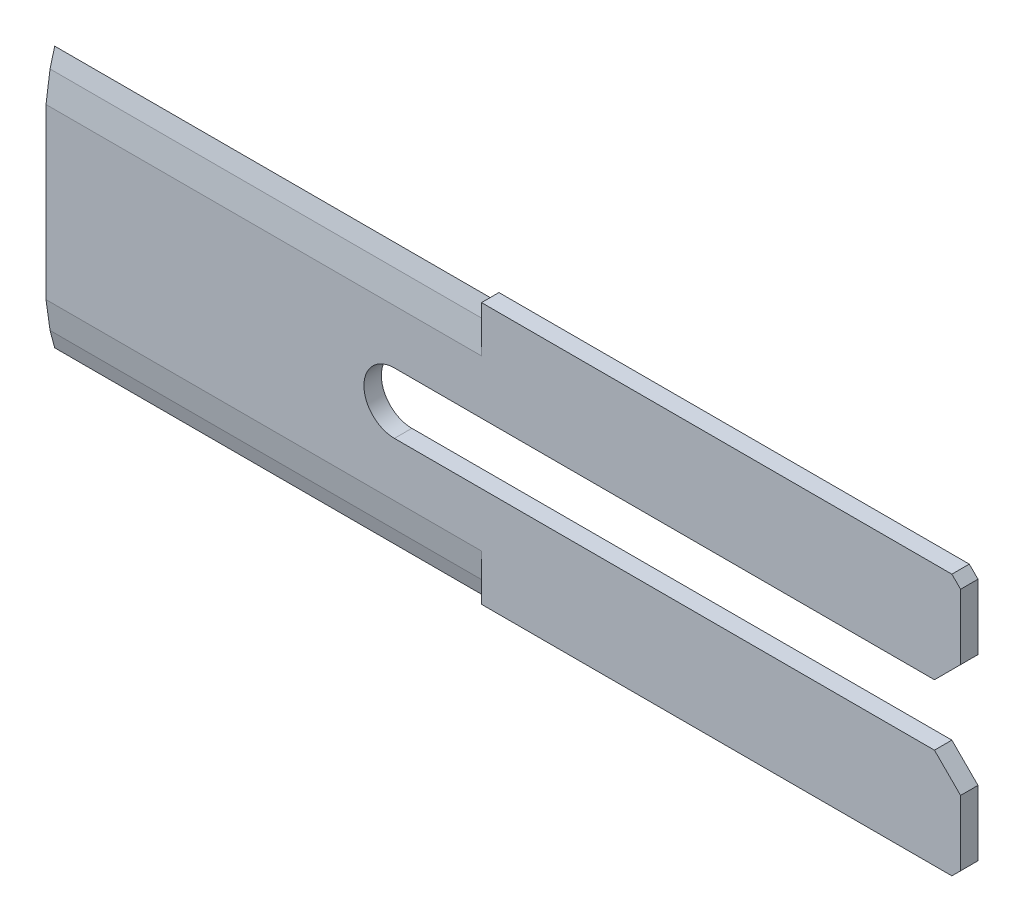
SolidWorks part; units mm, degrees
ref_plane "前视基准面" through (0, 0, 0) normal (0, 0, 1) x (1, 0, 0)
ref_plane "上视基准面" through (0, 0, 0) normal (0, 1, 0) x (1, 0, 0)
ref_plane "右视基准面" through (0, 0, 0) normal (1, 0, 0) x (0, 0, -1)
sketch "草图2" plane through (0, 0, 0) normal (0, 0, 1) x (1, 0, 0)
  line L1 (-52.5, 15) -> (52.5, 15)
  line L2 (-52.5, 15) -> (-52.5, -15)
  line L3 (-52.5, -15) -> (52.5, -15)
  line L4 (52.5, 15) -> (52.5, -15)
  line L5 (-52.5, 15) -> (52.5, -15) construction
  line L6 (-52.5, -15) -> (52.5, 15) construction
  point P0 (0, 0)
  dimension "D1" = 105
  dimension "D2" = 30
extrude "凸台-拉伸1" add sketch "草图2" along normal blind 2
sketch "草图3" plane through (0, 0, 2) normal (0, 0, 1) x (1, 0, 0)
  line L0 (-12.5, 3.5) -> (52.5, 3.5)
  line L1 (52.5, -15) -> (52.5, 15) construction
  line L2 (-12.5, -3.5) -> (52.5, -3.5)
  line L3 (52.5, 15) -> (-52.5, 15) construction
  arc A0 (-12.5, 3.5) -> (-12.5, -3.5) centre (-12.5, 0) ccw
  dimension "D1" = 7
  dimension "D2" = 65
  dimension "D3" = 15
extrude "切除-拉伸1" cut sketch "草图3" against normal through all and the other way through all
sketch "草图5" plane through (-52.5, 0, 0) normal (-1, 0, 0) x (0, 0, 1)
  line L0 (1, 16.6149) -> (1, -17.4095) construction
  line L1 (1, 15) -> (0.4641, 13)
  line L2 (2, 15) -> (0, 15) construction
  line L3 (1, 15) -> (1.5359, 13)
  line L4 (0, 9.6977) -> (0, -9.6977)
  line L5 (0.4641, 13) -> (0, 9.6977)
  line L6 (0, 15) -> (0, -15) construction
  line L7 (1.5359, 13) -> (2, 9.6977)
  line L8 (2, 15) -> (2, -15) construction
  line L9 (-0.6309, 0) -> (2.7776, 0) construction
  line L10 (1.5359, -13) -> (2, -9.6977)
  line L11 (0.4641, -13) -> (0, -9.6977)
  line L12 (2, -9.6977) -> (2, 9.6977)
  line L13 (1, -15) -> (1.5359, -13)
  line L14 (1, -15) -> (0.4641, -13)
  dimension "D1" = 30
  dimension "D2" = 15
  dimension "D4" = 2
  dimension "D5" = 16
  dimension "D6" = 8
extrude "切除-拉伸7" cut sketch "草图5" against normal blind 50 flip side to cut
chamfer "倒角1" distance 1 angle 45 2 edges at (52.5, -15, 1) (52.5, 15, 1)
chamfer "倒角2" distance 3 angle 45 2 edges at (52.5, 3.5, 1) (52.5, -3.5, 1)
